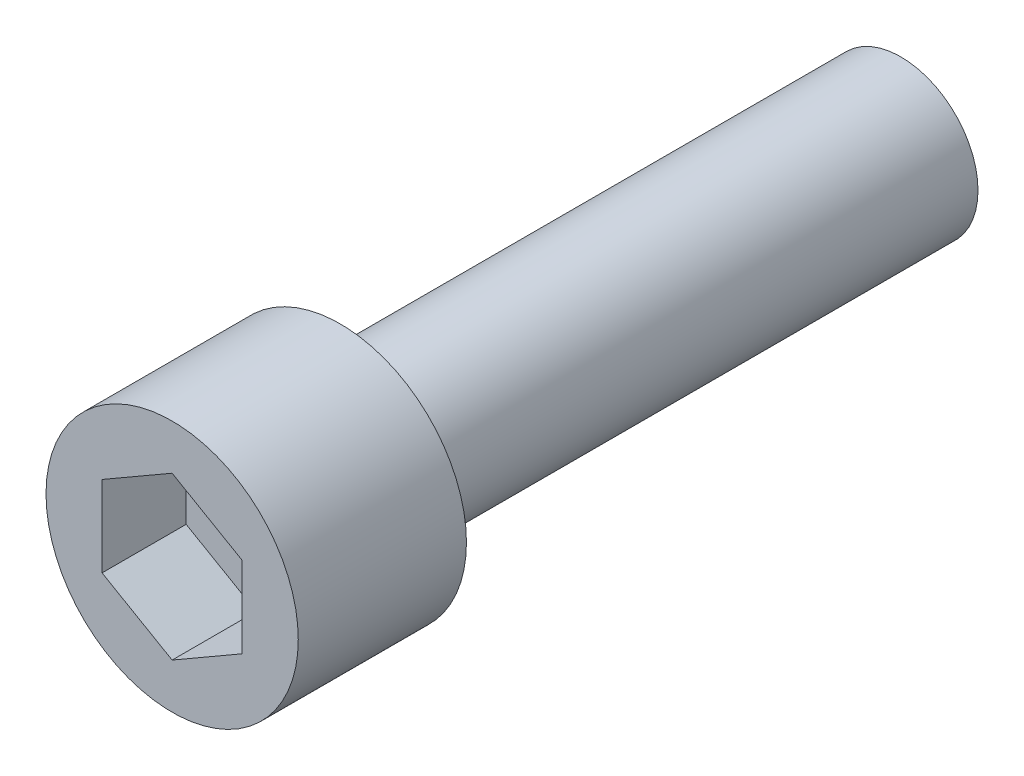
SolidWorks part; units mm, degrees
ref_plane "Front Plane" through (0, 0, 0) normal (0, 0, 1) x (1, 0, 0)
ref_plane "Top Plane" through (0, 0, 0) normal (0, 1, 0) x (1, 0, 0)
ref_plane "Right Plane" through (0, 0, 0) normal (1, 0, 0) x (0, 0, -1)
sketch "Sketch1" plane through (0, 0, 0) normal (0, 0, 1) x (1, 0, 0)
  circle A0 centre (0, 0) radius 5.5
extrude "Boss-Extrude1" add sketch "Sketch1" along normal blind 40
cosmetic thread "Cosmetic Thread1" parameters "D1"=32, "D2"=10
sketch "Sketch2" plane through (0, 0, 40) normal (0, 0, 1) x (1, 0, 0)
  circle A0 centre (0, 0) radius 9
extrude "Boss-Extrude2" add sketch "Sketch2" along normal blind 12
sketch "Sketch3" plane through (0, 0, 52) normal (0, 0, 1) x (1, 0, 0)
  line L1 (0, 5.7735) -> (-5, 2.8868)
  line L2 (-5, 2.8868) -> (-5, -2.8868)
  line L3 (-5, -2.8868) -> (0, -5.7735)
  line L4 (0, -5.7735) -> (5, -2.8868)
  line L5 (5, -2.8868) -> (5, 2.8868)
  line L6 (5, 2.8868) -> (0, 5.7735)
  circle A0 centre (0, 0) radius 5 construction
  dimension "D1" = 10
extrude "Cut-Extrude1" cut sketch "Sketch3" against normal blind 6 contours L1 L2 L3 L4 L5 L6
